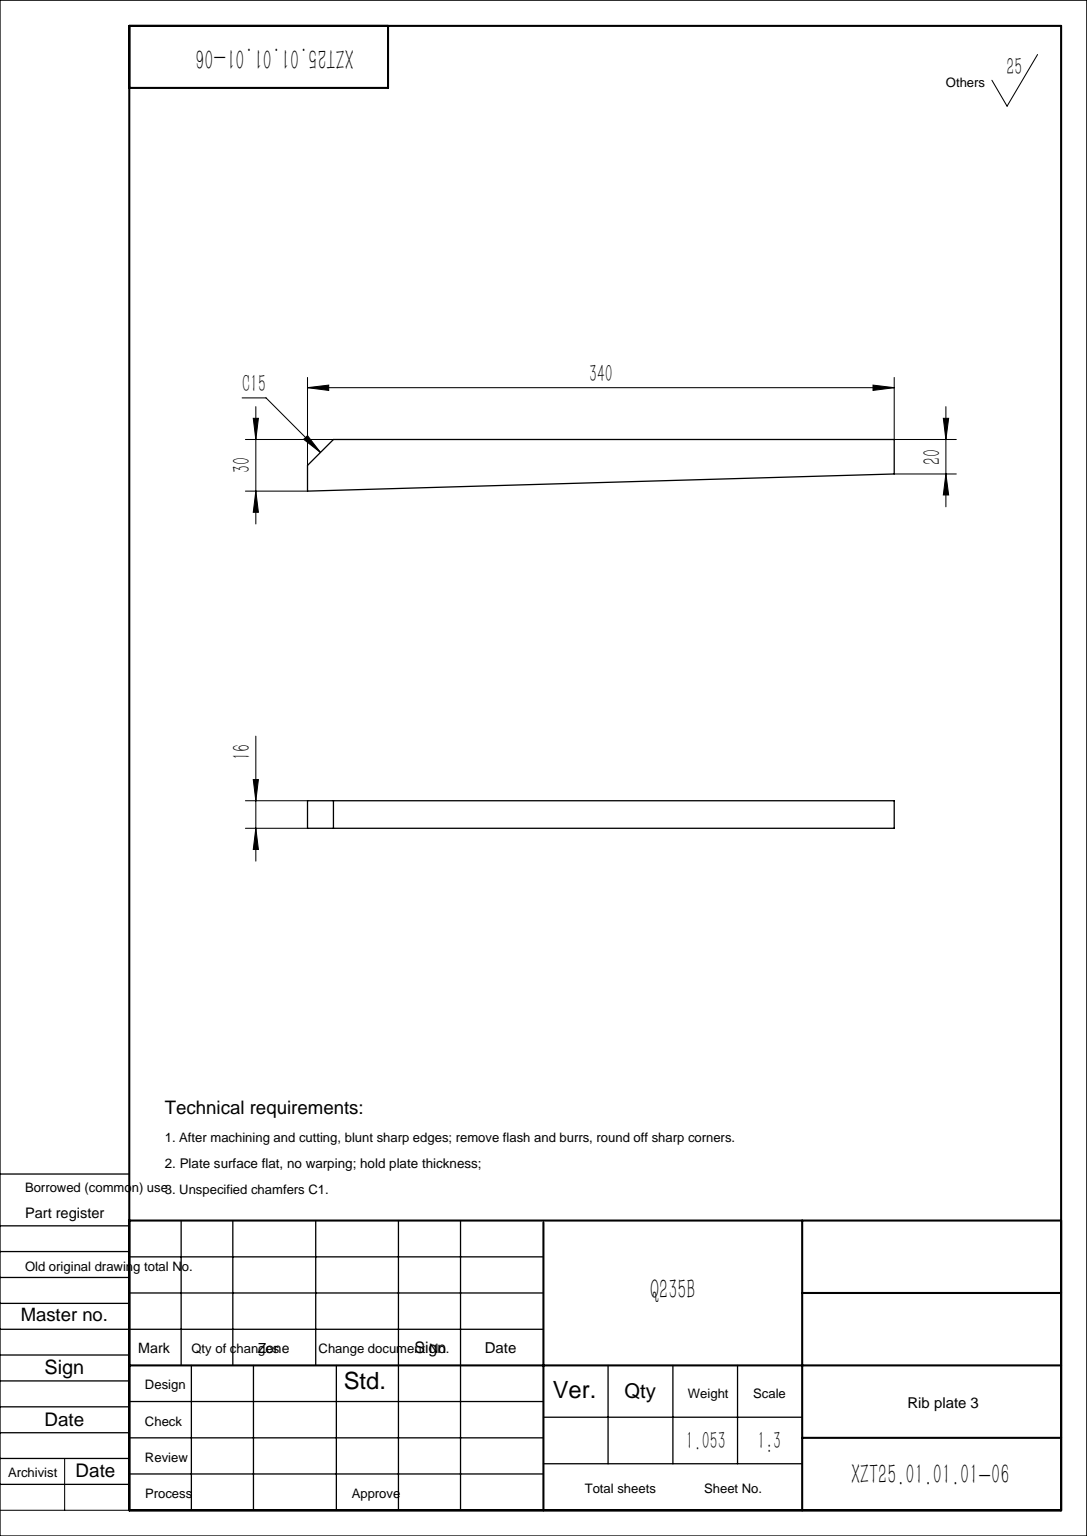
from build123d import *

# Parameters (mm, degrees)
BOSS_EXTRUDE1_DEPTH = 8
CHAMFER1_SIZE       = 15


with BuildPart() as part:
    # Sketch1 → Boss-Extrude1 (new, symmetric)
    with BuildSketch(Plane.XY):
        Polygon((0, 0), (0, 30), (340, 30), (340, 10), align=None)
    extrude(amount=BOSS_EXTRUDE1_DEPTH, both=True)

    # Chamfer1
    chamfer1_edges = [part.edges().sort_by_distance(p)[0] for p in [
        (0, 30, 0),
    ]]
    chamfer(chamfer1_edges, length=CHAMFER1_SIZE)


solid = part.part
